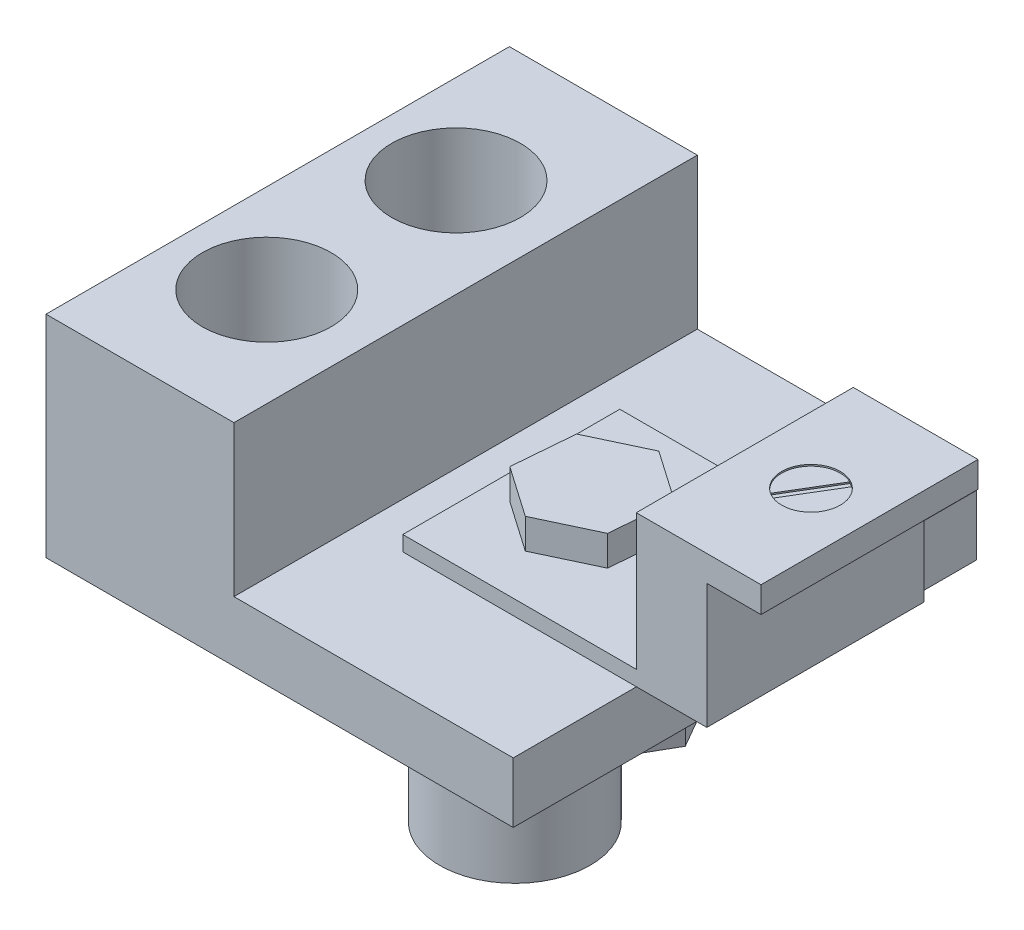
SolidWorks part; units mm, degrees
ref_plane "Front Plane" through (0, 0, 0) normal (0, 0, 1) x (1, 0, 0)
ref_plane "Top Plane" through (0, 0, 0) normal (0, 1, 0) x (1, 0, 0)
ref_plane "Right Plane" through (0, 0, 0) normal (1, 0, 0) x (0, 0, -1)
sketch "Sketch1" plane through (0, 0, 0) normal (0, 1, 0) x (1, 0, 0)
  line L1 (5.7735, 10) -> (-5.7735, 10)
  line L2 (-5.7735, 10) -> (-11.547, 0)
  line L3 (-11.547, 0) -> (-5.7735, -10)
  line L4 (-5.7735, -10) -> (5.7735, -10)
  line L5 (5.7735, -10) -> (11.547, 0)
  line L6 (11.547, 0) -> (5.7735, 10)
  circle A0 centre (0, 0) radius 10 construction
  dimension "D1" = 20
extrude "Boss-Extrude1" add sketch "Sketch1" along normal blind 5
sketch "Sketch2" plane through (0, 0, 0) normal (0, -1, 0) x (1, 0, 0)
  circle A0 centre (0.2348, 0) radius 5
  dimension "D1" = 10
extrude "Boss-Extrude2" add sketch "Sketch2" along normal blind 10
sketch "Sketch3" plane through (0, 5, 0) normal (0, 1, 0) x (1, 0, 0)
  line L1 (-15.5042, -15.376) -> (15.5042, -15.376)
  line L2 (-15.5042, -15.376) -> (-15.5042, 15.376)
  line L3 (-15.5042, 15.376) -> (15.5042, 15.376)
  line L4 (15.5042, -15.376) -> (15.5042, 15.376)
  line L5 (-15.5042, -15.376) -> (15.5042, 15.376) construction
  line L6 (-15.5042, 15.376) -> (15.5042, -15.376) construction
  point P0 (0, 0)
extrude "Boss-Extrude3" add sketch "Sketch3" along normal blind 4
sketch "Sketch4" plane through (0, 9, 0) normal (0, 1, 0) x (1, 0, 0)
  line L0 (-15.5042, -15.376) -> (15.5042, -15.376) construction
  line L1 (-15.5042, 15.376) -> (-3.0312, 15.376)
  line L2 (-15.5042, 15.376) -> (-15.5042, -15.376)
  line L3 (-15.5042, -15.376) -> (-3.0312, -15.376)
  line L4 (-3.0312, 15.376) -> (-3.0312, -15.376)
  line L5 (15.5042, 15.376) -> (-15.5042, 15.376) construction
extrude "Boss-Extrude4" add sketch "Sketch4" along normal blind 10
sketch "Sketch5" plane through (0, 9, 0) normal (0, 1, 0) x (1, 0, 0)
  line L1 (0, 7.2005) -> (20.1802, 7.2005)
  line L2 (0, 7.2005) -> (0, -7.2005)
  line L3 (0, -7.2005) -> (20.1802, -7.2005)
  line L4 (20.1802, 7.2005) -> (20.1802, -7.2005)
  line L5 (0, 7.2005) -> (20.1802, -7.2005) construction
  line L6 (0, -7.2005) -> (20.1802, 7.2005) construction
  point P0 (10.0901, 0)
extrude "Boss-Extrude5" add sketch "Sketch5" along normal blind 1
sketch "Sketch6" plane through (0, 0, 7.2005) normal (0, 0, 1) x (1, 0, 0)
  line L0 (20.1802, 10) -> (20.1802, 17.284)
  line L1 (20.1802, 17.284) -> (23.7726, 17.284)
  line L2 (23.7726, 17.284) -> (23.7726, 19)
  line L3 (23.7726, 19) -> (15.4949, 19)
  line L4 (-15.5042, 19) -> (-3.0312, 19) construction
  line L5 (20.1802, 10) -> (15.4949, 10)
  line L6 (0, 10) -> (20.1802, 10) construction
  line L7 (15.4949, 10) -> (15.4949, 19)
extrude "Boss-Extrude6" add sketch "Sketch6" against normal up to surface (14.4009 mm away) up to face at (11.1729, 9.4, -7.2005)
sketch "Sketch7" plane through (0, 19, 0) normal (0, 1, 0) x (1, 0, 0)
  circle A0 centre (-9.5837, 5.9173) radius 4.271
  circle A1 centre (-9.5837, -6.6455) radius 4.271
extrude "Cut-Extrude1" cut sketch "Sketch7" against normal blind 11
sketch "Sketch8" plane through (0, 19, 0) normal (0, 1, 0) x (1, 0, 0)
  circle A0 centre (19.8895, 0) radius 1.943
extrude "Cut-Extrude2" cut sketch "Sketch8" against normal blind 0.1
sketch "Sketch9" plane through (0, 18.9, 0) normal (0, 1, 0) x (1, 0, 0)
  line L0 (18.7142, -1.5607) -> (20.7141, 1.7712)
  line L1 (18.7142, -1.5607) -> (19.0649, -1.7712)
  line L2 (20.7141, 1.7712) -> (21.0648, 1.5607)
  line L3 (19.0649, -1.7712) -> (21.0648, 1.5607)
  line L4 (18.7142, -1.5607) -> (21.0648, 1.5607) construction
  line L5 (20.7141, 1.7712) -> (19.0649, -1.7712) construction
  point P1 (19.8895, 0)
extrude "Cut-Extrude3" cut sketch "Sketch9" against normal blind 0.1
sketch "Sketch10" plane through (0, 10, 0) normal (0, 1, 0) x (1, 0, 0)
  line L1 (5.7033, 4.089) -> (1.991, 2.3409)
  line L2 (1.991, 2.3409) -> (1.6488, -1.7481)
  line L3 (1.6488, -1.7481) -> (5.0188, -4.089)
  line L4 (5.0188, -4.089) -> (8.7311, -2.3409)
  line L5 (8.7311, -2.3409) -> (9.0733, 1.7481)
  line L6 (9.0733, 1.7481) -> (5.7033, 4.089)
  circle A0 centre (5.361, 0) radius 3.5535 construction
extrude "Boss-Extrude7" add sketch "Sketch10" along normal blind 2
